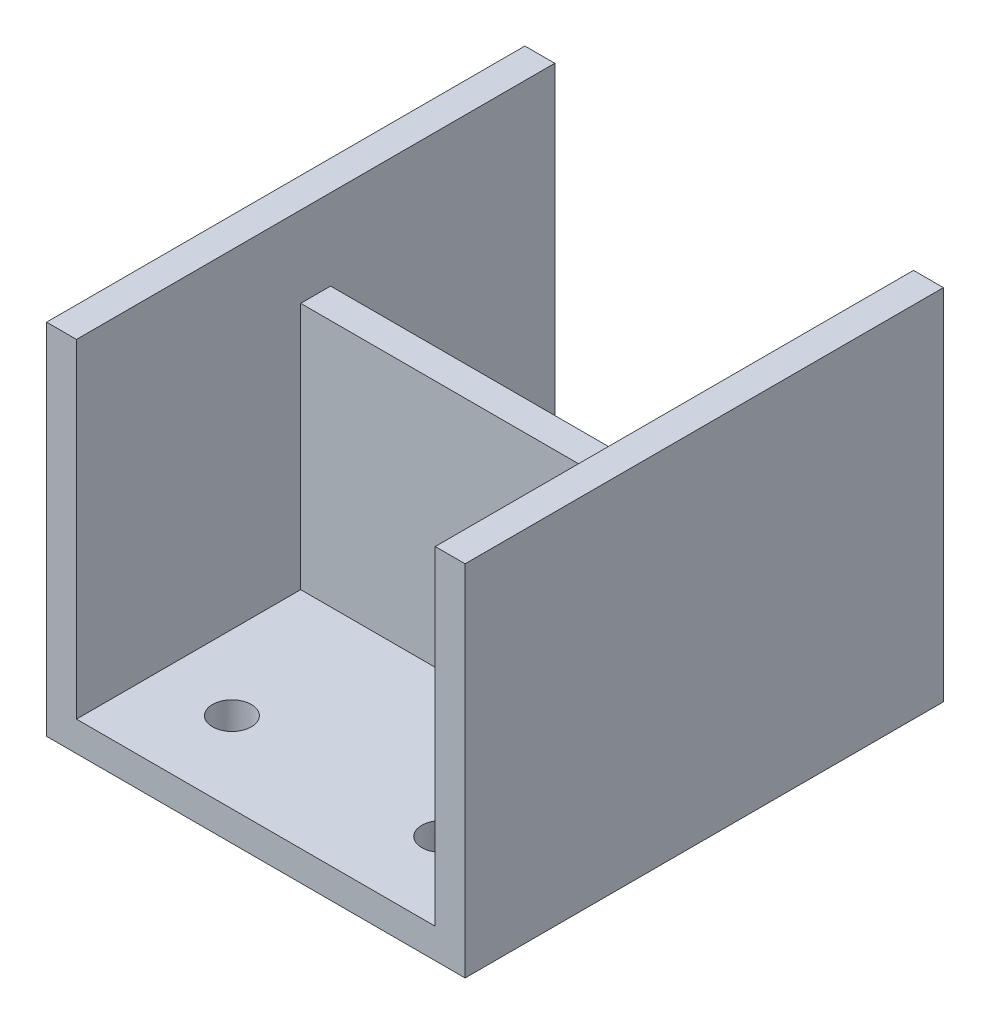
SolidWorks part; units mm, degrees
material "1023 碳钢板 (SS)"
ref_plane "前视基准面" through (0, 0, 0) normal (0, 0, 1) x (1, 0, 0)
ref_plane "上视基准面" through (0, 0, 0) normal (0, 1, 0) x (1, 0, 0)
ref_plane "右视基准面" through (0, 0, 0) normal (1, 0, 0) x (0, 0, -1)
sketch "草图1" plane through (0, 0, 0) normal (0, 0, 1) x (1, 0, 0)
  line L0 (-30, 30) -> (-30, -25)
  line L1 (35, -30) -> (-35, -30)
  line L2 (35, -30) -> (35, 30)
  line L3 (35, 30) -> (30, 30)
  line L4 (-35, -30) -> (-35, 30)
  line L5 (35, -30) -> (-35, 30) construction
  line L6 (35, 30) -> (-35, -30) construction
  line L7 (-30, -25) -> (30, -25)
  line L8 (30, -25) -> (30, 30)
  line L9 (-30, 30) -> (-35, 30)
  point P0 (0, 0)
  dimension "D1" = 70
  dimension "D2" = 60
  dimension "D3" = 5
  dimension "D4" = 5
  dimension "D5" = 5
extrude "凸台-拉伸1" add sketch "草图1" along normal mid plane 80
sketch "草图2" plane through (0, 0, 0) normal (0, 0, 1) x (1, 0, 0)
  line L0 (30, 30) -> (30, -25) construction
  line L1 (-30, -25) -> (30, -25)
  line L2 (-30, -25) -> (-30, 16.4763)
  line L3 (-30, 16.4763) -> (30, 16.4763)
  line L4 (30, -25) -> (30, 16.4763)
extrude "凸台-拉伸2" add sketch "草图2" along normal mid plane 5
sketch "草图3" plane through (0, -30, 0) normal (0, -1, 0) x (1, 0, 0)
  circle A0 centre (17.5, 26.5) radius 3.25
  circle A1 centre (17.5, -8.5) radius 3.25
  circle A2 centre (-17.5, -8.5) radius 3.25
  circle A3 centre (-17.5, 26.5) radius 3.25
  dimension "D1" = 6.5
extrude "切除-拉伸1" cut sketch "草图3" against normal blind 10
